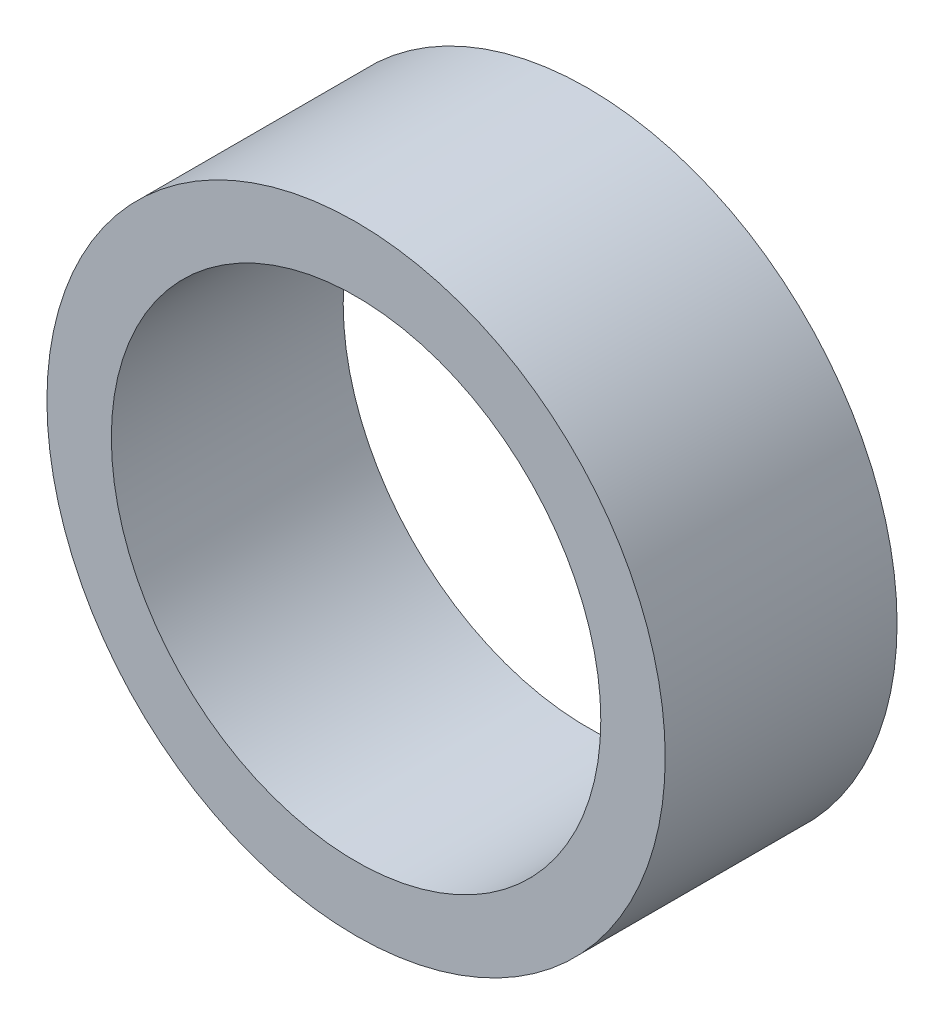
from build123d import *

# Parameters (mm, degrees)
SKETCH_1_R      = 24
SKETCH_1_R_2    = 19
EXTRUDE_1_DEPTH = 18


with BuildPart() as part:
    # 草图1 → 凸台-拉伸1 (new body)
    with BuildSketch(Plane.XY):
        Circle(SKETCH_1_R)
        Circle(SKETCH_1_R_2, mode=Mode.SUBTRACT)
    extrude(amount=EXTRUDE_1_DEPTH)


solid = part.part
